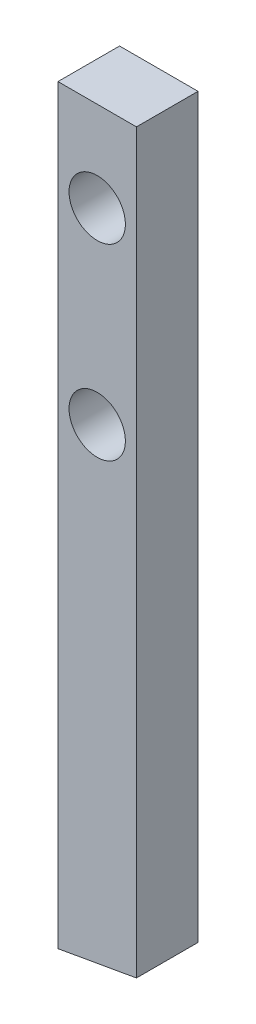
SolidWorks part; units mm, degrees
ref_plane "Front Plane" through (0, 0, 0) normal (0, 0, 1) x (1, 0, 0)
ref_plane "Top Plane" through (0, 0, 0) normal (0, 1, 0) x (1, 0, 0)
ref_plane "Right Plane" through (0, 0, 0) normal (1, 0, 0) x (0, 0, -1)
sketch "Sketch1" plane through (0, 0, 0) normal (0, 1, 0) x (1, 0, 0)
  line L8 (-2.09, 1.64) -> (-2.09, -1.64)
  line L11 (-2.09, -1.64) -> (2.09, -1.64)
  line L14 (2.09, -1.64) -> (2.09, 1.64)
  line L15 (2.09, 1.64) -> (-2.09, 1.64)
  dimension "D2" = 4.18
  dimension "D1" = 3.28
extrude "Boss-Extrude1" add sketch "Sketch1" along normal blind 40
sketch "Sketch2" plane through (0, 0, 1.64) normal (0, 0, 1) x (1, 0, 0)
  line L0 (-2.09, 0) -> (2.09, 0)
  line L3 (-2.09, 0) -> (2.09, 0) construction
  line L4 (2.09, 0) -> (2.09, 0.737)
  line L5 (2.09, 40) -> (2.09, 0) construction
  line L6 (2.09, 0.737) -> (-2.09, 0)
  dimension "D1" = 10
extrude "Cut-Extrude1" cut sketch "Sketch2" against normal blind 40
sketch "Sketch3" plane through (0, 0, -1.64) normal (0, 0, -1) x (-1, 0, 0)
  circle A0 centre (0, 35.2112) radius 1.5
  circle A1 centre (0, 25.2112) radius 1.5
  dimension "D1" = 3
  dimension "D2" = 3
  dimension "D3" = 10
extrude "Cut-Extrude2" cut sketch "Sketch3" against normal blind 40
